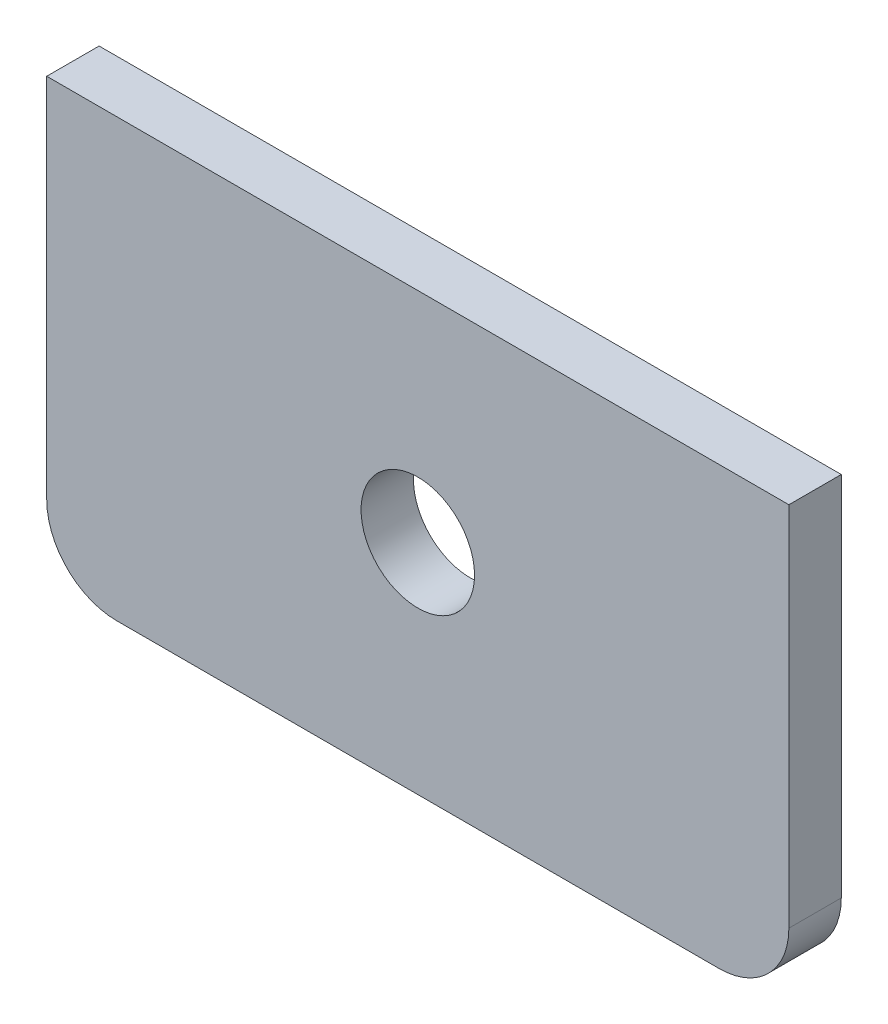
from build123d import *

# Parameters (mm, degrees)
SKETCH_1_R      = 6.5
EXTRUDE_1_DEPTH = 6


with BuildPart() as part:
    # 草图1 → 凸台-拉伸1 (new body)
    with BuildSketch(Plane.XY):
        with BuildLine():
            Line((-42.5, 25), (42.5, 25))
            Line((42.5, 25), (42.5, -17))
            ThreePointArc((42.5, -17), (40.156854249, -22.656854249), (34.5, -25))
            Line((34.5, -25), (-34.5, -25))
            ThreePointArc((-34.5, -25), (-40.156854249, -22.656854249), (-42.5, -17))
            Line((-42.5, -17), (-42.5, 25))
        make_face()
        Circle(SKETCH_1_R, mode=Mode.SUBTRACT)
    extrude(amount=EXTRUDE_1_DEPTH)


solid = part.part
